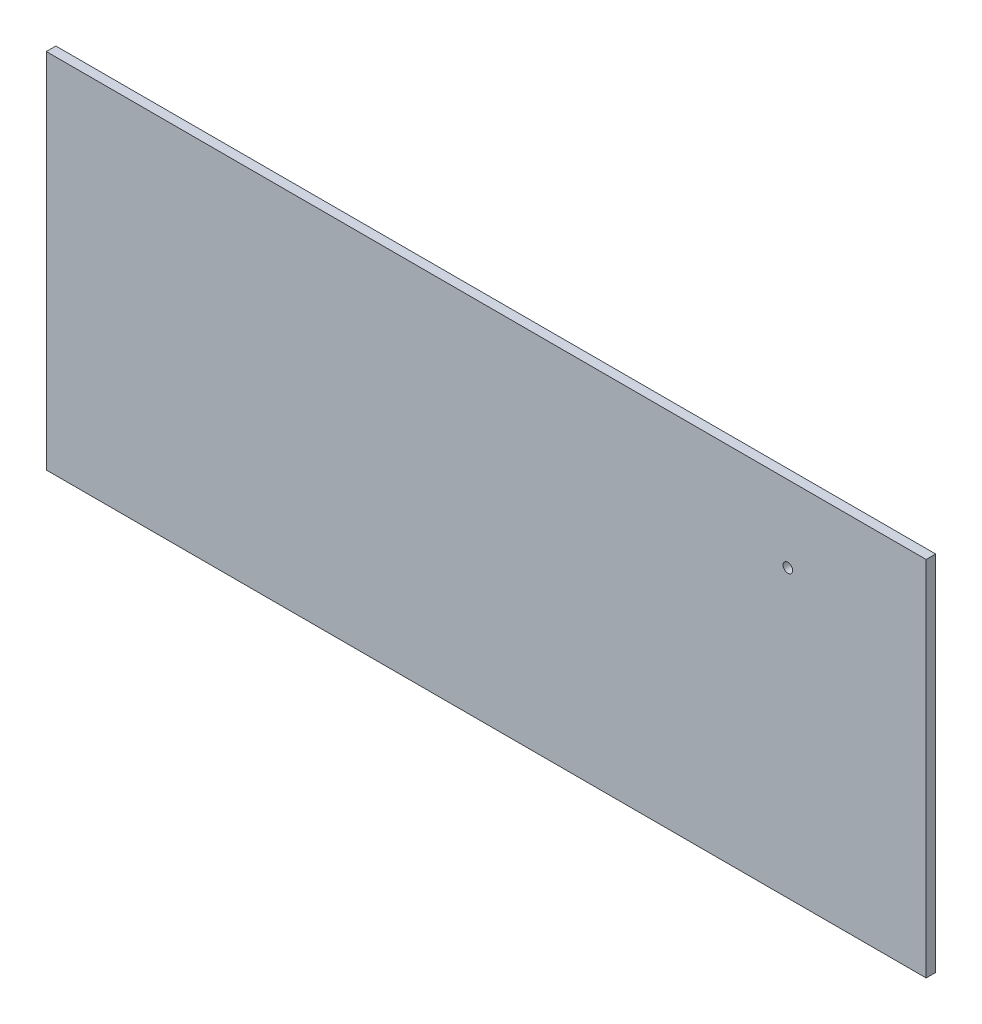
SolidWorks part; units mm, degrees
material "Q235"
ref_plane "Front Plane" through (0, 0, 0) normal (0, 0, 1) x (1, 0, 0)
ref_plane "Top Plane" through (0, 0, 0) normal (0, 1, 0) x (1, 0, 0)
ref_plane "Right Plane" through (0, 0, 0) normal (1, 0, 0) x (0, 0, -1)
sketch "Sketch1" plane through (0, 0, 0) normal (0, 0, 1) x (1, 0, 0)
  line L1 (0, 0) -> (1845, 0)
  line L2 (0, 0) -> (0, 760)
  line L3 (0, 760) -> (1845, 760)
  line L4 (1845, 0) -> (1845, 760)
  circle A0 centre (1555, 600) radius 10
  dimension "D3" = 290
  dimension "D4" = 160
  dimension "D5" = 20
  dimension "D1" = 1845
  dimension "D2" = 760
extrude "Boss-Extrude1" add sketch "Sketch1" along normal blind 20
